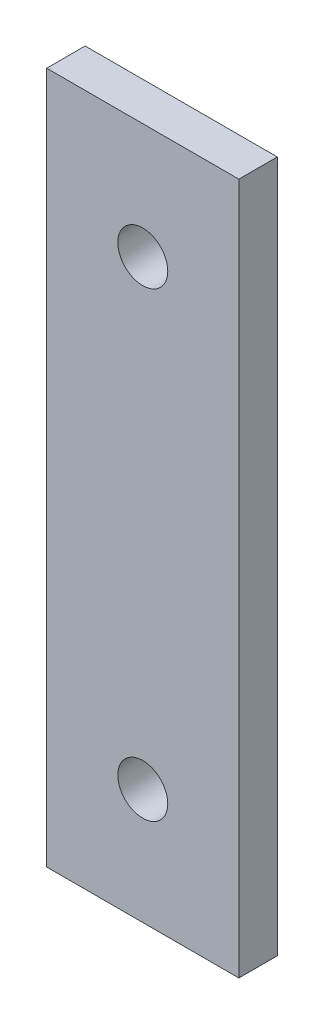
from build123d import *

# Parameters (mm, degrees)
SKETCH_1_W          = 50
SKETCH_1_H          = 180
EXTRUDE_1_DEPTH     = 10
SKETCH_2_R          = 6.5
CUT_EXTRUDE_1_DEPTH = 10


with BuildPart() as part:
    # 草图1 → 凸台-拉伸1 (new body)
    with BuildSketch(Plane.XY):
        with Locations((25, 90)):
            Rectangle(SKETCH_1_W, SKETCH_1_H)
    extrude(amount=EXTRUDE_1_DEPTH)

    # 草图2 → 切除-拉伸1 (cut)
    with BuildSketch(Plane.XY.offset(10)):
        with Locations((25, 150)):
            Circle(SKETCH_2_R)
        with Locations((25, 30)):
            Circle(SKETCH_2_R)
    extrude(amount=-CUT_EXTRUDE_1_DEPTH, mode=Mode.SUBTRACT)


solid = part.part
